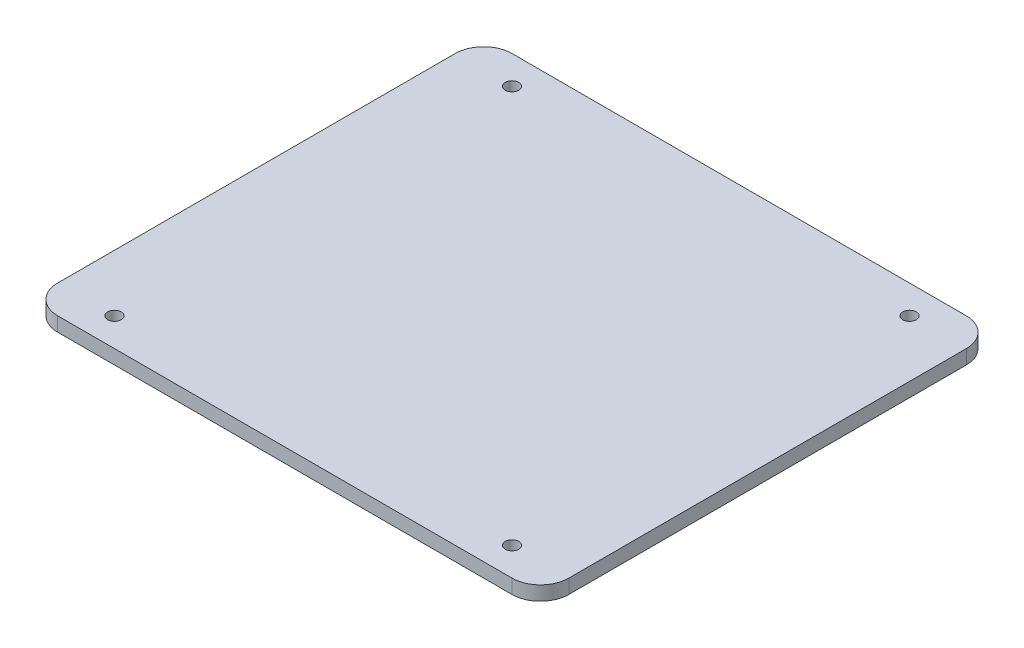
SolidWorks part; units mm, degrees
material "透明亚克力"
ref_plane "Front Plane" through (0, 0, 0) normal (0, 0, 1) x (1, 0, 0)
ref_plane "Top Plane" through (0, 0, 0) normal (0, 1, 0) x (1, 0, 0)
ref_plane "Right Plane" through (0, 0, 0) normal (1, 0, 0) x (0, 0, -1)
sketch "Sketch1" plane through (0, 0, 0) normal (0, 1, 0) x (1, 0, 0)
  line L1 (-90, 80) -> (90, 80)
  line L2 (-90, 80) -> (-90, -80)
  line L3 (-90, -80) -> (90, -80)
  line L4 (90, 80) -> (90, -80)
  line L5 (-90, 80) -> (90, -80) construction
  line L6 (-90, -80) -> (90, 80) construction
  point P0 (0, 0)
  dimension "D1" = 180
  dimension "D2" = 160
extrude "Boss-Extrude1" add sketch "Sketch1" along normal mid plane 5
sketch "Sketch2" plane through (0, 2.5, 0) normal (0, 1, 0) x (1, 0, 0)
  line L0 (90, 80) -> (-90, 80) construction
  line L1 (-70, 70) -> (70, 70) construction
  line L2 (-70, 70) -> (-70, -70) construction
  line L3 (-70, -70) -> (70, -70) construction
  line L4 (70, 70) -> (70, -70) construction
  line L5 (-70, 70) -> (70, -70) construction
  line L6 (-70, -70) -> (70, 70) construction
  line L7 (90, -80) -> (90, 80) construction
  point P0 (0, 0)
  dimension "D1" = 10
  dimension "D2" = 20
hole_wizard "M4 Clearance Hole1" positions "3DSketch1" profile "Sketch3" hole size "M4" standard "GB" end condition up to next
sketch3d "3DSketch1"
  point P0 (-70, 2.5, -70)
  point P3 (70, 2.5, -70)
  point P6 (70, 2.5, 70)
  point P9 (-70, 2.5, 70)
sketch "Sketch3" plane through (-70, 2.5, -70) normal (1, 0, 0) x (0, 0, 1)
  line L0 (0, 0) -> (0, 5)
  line L1 (0, 5) -> (2.4, 5)
  line L2 (2.4, 5) -> (2.4, 0)
  line L5 (2.4, 0) -> (0, 0)
  line L11 (0, -6.35) -> (0, 107.95) construction
  dimension "通孔孔直径" = 4.8
  dimension "通孔孔深度" = 5
fillet "Fillet1" radius 10 4 edges at (90, 0, 80) (-90, 0, 80) (90, 0, -80) (-90, 0, -80)
